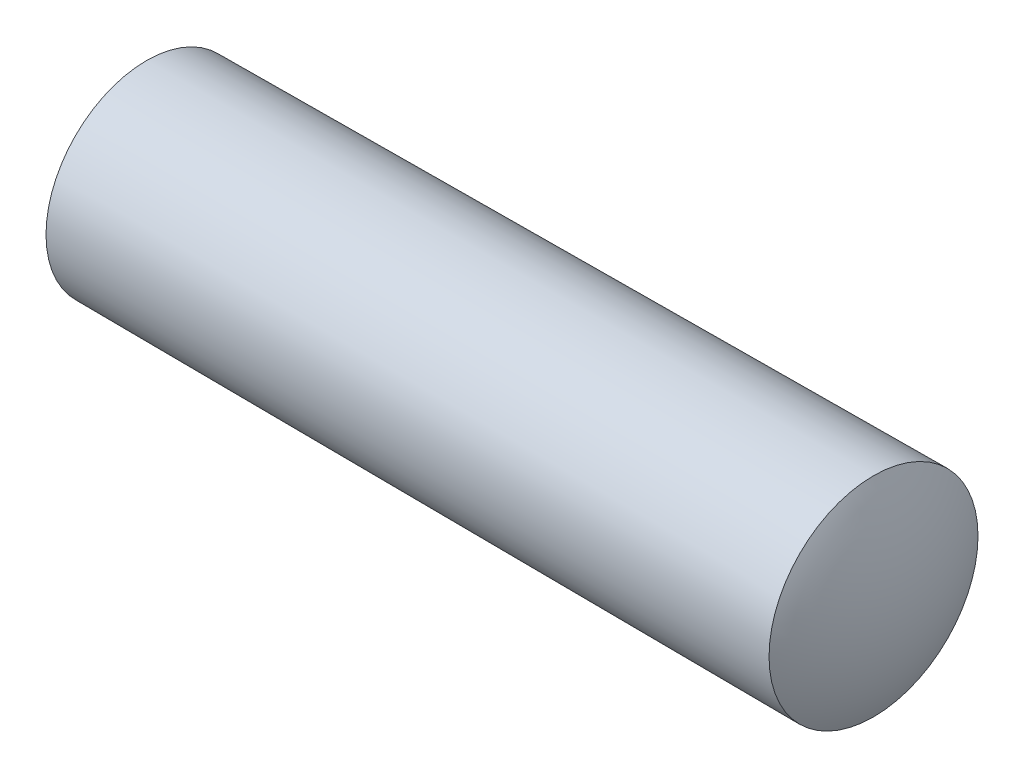
SolidWorks part; units mm, degrees
ref_plane "Front Plane" through (0, 0, 0) normal (0, 0, 1) x (1, 0, 0)
ref_plane "Top Plane" through (0, 0, 0) normal (0, 1, 0) x (1, 0, 0)
ref_plane "Right Plane" through (0, 0, 0) normal (1, 0, 0) x (0, 0, -1)
sketch "Sketch1" plane through (0, 0, 0) normal (0, 0, 1) x (1, 0, 0)
  line L0 (-7, 3.873) -> (21, 4.0241)
  line L1 (-8, 0) -> (22, 0)
  arc A0 (-7, 3.873) -> (-8, 0) centre (0, 0) ccw
  arc A1 (22, 0) -> (21, 4.0241) centre (13.4032, 0) ccw
revolve "Revolve1" add sketch "Sketch1" angle 360 about L1
equation "\"d\"= 8'公称直径"
equation "\"a\"= 1"
equation "\"l\"= 30'公称长度"
equation "\"r1\"= \"d\""
equation "\"r2\"= \"a\" / 2 + \"d\" + sqr ( 0.02 * \"l\" ) / ( 8 * \"a\" )"
equation "\"D1@Sketch1\"=\"l\""
equation "\"D2@Sketch1\"=\"r1\""
equation "\"D3@Sketch1\"=\"a\""
equation "\"D4@Sketch1\"=\"r2\""
equation "\"D5@Sketch1\"=\"a\""
